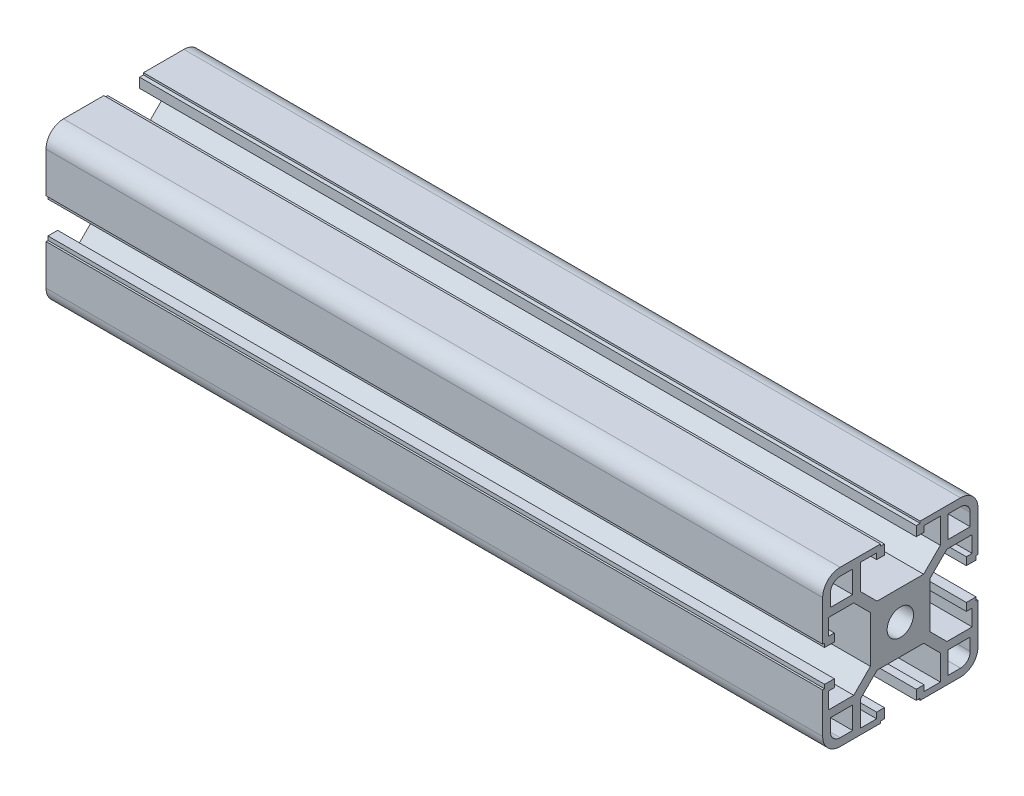
SolidWorks part; units mm, degrees
ref_plane "Front Plane" through (0, 0, 0) normal (0, 0, 1) x (1, 0, 0)
ref_plane "Top Plane" through (0, 0, 0) normal (0, 1, 0) x (1, 0, 0)
ref_plane "Right Plane" through (0, 0, 0) normal (1, 0, 0) x (0, 0, -1)
sketch "草图1" plane through (0, 0, 0) normal (0, 0, 1) x (1, 0, 0)
  line L0 (-984.975, 0) -> (-784.975, 0)
  dimension "D1" = 200
other "Aluminium profile 40 X 40B X R4.5(1)"
ref_plane "Plane1" through (-984.975, 0, 0) normal (1, 0, 0) x (0, 1, 0)
sketch "Sketch1" plane through (-984.975, 0, 0) normal (1, 0, 0) x (0, 1, 0)
  line L0 (-5.1, 20) -> (-5.1, 19.5)
  line L1 (-5.1, 19.5) -> (-4.1, 19.5)
  line L2 (-4.1, 19.5) -> (-4.1, 17)
  line L3 (-6.1, 18.5) -> (-10.3, 18.5)
  line L4 (-15.5, -20) -> (-5.1, -20)
  line L5 (-20, -15.5) -> (-20, -5.1)
  line L6 (15.5, 20) -> (5.1, 20)
  line L7 (20, 15.5) -> (20, 5.1)
  line L8 (0, 14.8756) -> (0, 0) construction
  line L9 (0, 0) -> (14.1675, 0) construction
  line L10 (-10.3, 18.5) -> (-10.3, 12)
  line L11 (-10.3, 12) -> (-6, 7.7)
  line L12 (-6, 7.7) -> (6, 7.7)
  line L13 (10.3, 12) -> (6, 7.7)
  line L14 (10.3, 18.5) -> (10.3, 12)
  line L15 (6.1, 18.5) -> (10.3, 18.5)
  line L16 (4.1, 19.5) -> (4.1, 17)
  line L17 (5.1, 19.5) -> (4.1, 19.5)
  line L18 (5.1, 20) -> (5.1, 19.5)
  line L19 (-5.1, 20) -> (-15.5, 20)
  line L20 (20, 5.1) -> (19.5, 5.1)
  line L21 (12.3, 18) -> (15.5, 18)
  line L22 (12.3, 18) -> (12.3, 12.3)
  line L23 (12.3, 12.3) -> (18, 12.3)
  line L24 (18, 15.5) -> (18, 12.3)
  line L25 (19.5, 5.1) -> (19.5, 4.1)
  line L26 (19.5, 4.1) -> (17, 4.1)
  line L27 (17, 6.1) -> (17, 4.1)
  line L28 (18.5, 6.1) -> (17, 6.1)
  line L29 (18.5, 6.1) -> (18.5, 10.3)
  line L30 (18.5, 10.3) -> (12, 10.3)
  line L31 (12, 10.3) -> (7.7, 6)
  line L32 (7.7, 6) -> (7.7, -6)
  line L33 (12, -10.3) -> (7.7, -6)
  line L34 (18.5, -10.3) -> (12, -10.3)
  line L35 (18.5, -6.1) -> (18.5, -10.3)
  line L36 (18.5, -6.1) -> (17, -6.1)
  line L37 (17, -4.1) -> (17, -6.1)
  line L38 (19.5, -4.1) -> (17, -4.1)
  line L39 (19.5, -5.1) -> (19.5, -4.1)
  line L40 (20, -5.1) -> (19.5, -5.1)
  line L41 (5.1, -20) -> (5.1, -19.5)
  line L42 (5.1, -19.5) -> (4.1, -19.5)
  line L43 (4.1, -19.5) -> (4.1, -17)
  line L44 (6.1, -17) -> (4.1, -17)
  line L45 (6.1, -18.5) -> (6.1, -17)
  line L46 (6.1, -18.5) -> (10.3, -18.5)
  line L47 (10.3, -18.5) -> (10.3, -12)
  line L48 (10.3, -12) -> (6, -7.7)
  line L49 (6, -7.7) -> (-6, -7.7)
  line L50 (-10.3, -12) -> (-6, -7.7)
  line L51 (-10.3, -18.5) -> (-10.3, -12)
  line L52 (-6.1, -18.5) -> (-10.3, -18.5)
  line L53 (-6.1, -18.5) -> (-6.1, -17)
  line L54 (-4.1, -17) -> (-6.1, -17)
  line L55 (-4.1, -19.5) -> (-4.1, -17)
  line L56 (-5.1, -19.5) -> (-4.1, -19.5)
  line L57 (-5.1, -20) -> (-5.1, -19.5)
  line L58 (-20, -5.1) -> (-19.5, -5.1)
  line L59 (5.1, -20) -> (15.5, -20)
  line L60 (-20, 5.1) -> (-20, 15.5)
  line L61 (-19.5, -5.1) -> (-19.5, -4.1)
  line L62 (-6.1, 18.5) -> (-6.1, 17)
  line L63 (-6.1, 17) -> (-4.1, 17)
  line L64 (6.1, 18.5) -> (6.1, 17)
  line L65 (4.1, 17) -> (6.1, 17)
  line L66 (-19.5, -4.1) -> (-17, -4.1)
  line L67 (-15.5, 18) -> (-12.3, 18)
  line L68 (-18, 15.5) -> (-18, 12.3)
  line L69 (-18, 12.3) -> (-12.3, 12.3)
  line L70 (-12.3, 18) -> (-12.3, 12.3)
  line L71 (-17, -6.1) -> (-17, -4.1)
  line L72 (-18.5, -6.1) -> (-17, -6.1)
  line L73 (-18.5, -6.1) -> (-18.5, -10.3)
  line L74 (-18.5, -10.3) -> (-12, -10.3)
  line L75 (-12, -10.3) -> (-7.7, -6)
  line L76 (-7.7, -6) -> (-7.7, 6)
  line L77 (-12, 10.3) -> (-7.7, 6)
  line L78 (-18.5, 10.3) -> (-12, 10.3)
  line L79 (-18.5, 6.1) -> (-18.5, 10.3)
  line L80 (-18.5, 6.1) -> (-17, 6.1)
  line L81 (-17, 4.1) -> (-17, 6.1)
  line L82 (-19.5, 4.1) -> (-17, 4.1)
  line L83 (-19.5, 5.1) -> (-19.5, 4.1)
  line L84 (-20, 5.1) -> (-19.5, 5.1)
  line L85 (20, -5.1) -> (20, -15.5)
  line L87 (-18, -12.3) -> (-12.3, -12.3)
  line L88 (-18, -12.3) -> (-18, -15.5)
  line L89 (-15.5, -18) -> (-12.3, -18)
  line L90 (-12.3, -12.3) -> (-12.3, -18)
  line L91 (12.3, -12.3) -> (18, -12.3)
  line L92 (12.3, -12.3) -> (12.3, -18)
  line L93 (12.3, -18) -> (15.5, -18)
  line L94 (18, -12.3) -> (18, -15.5)
  circle A0 centre (0, 0) radius 3.4
  arc A1 (-20, 15.5) -> (-15.5, 20) centre (-15.5, 15.5) cw
  arc A2 (20, 15.5) -> (15.5, 20) centre (15.5, 15.5) ccw
  arc A3 (-15.5, -20) -> (-20, -15.5) centre (-15.5, -15.5) cw
  arc A4 (15.5, -20) -> (20, -15.5) centre (15.5, -15.5) ccw
  arc A5 (-15.5, 18) -> (-18, 15.5) centre (-15.5, 15.5) ccw
  arc A6 (18, 15.5) -> (15.5, 18) centre (15.5, 15.5) ccw
  arc A7 (18, -15.5) -> (15.5, -18) centre (15.5, -15.5) cw
  arc A8 (-18, -15.5) -> (-15.5, -18) centre (-15.5, -15.5) ccw
  point P2 (0, 10)
  point P4 (0, 0)
  point P5 (-20, -20)
  point P6 (20, -20)
  point P7 (20, 20)
  point P8 (-20, 20)
  point P36 (-20, 20)
  point P39 (20, 20)
  point P121 (0, 0)
  dimension "D1" = 20.6
  dimension "D2" = 40
  dimension "D3" = 8.2
  dimension "D4" = 10.2
  dimension "D5" = 12.3
  dimension "D6" = 6.8
  dimension "D7" = 4.5
  dimension "D8" = 45
  dimension "D12" = 2
  dimension "D13" = 5.7
  dimension "D14" = 2
  dimension "D18" = 2.5
  dimension "D19" = 2.5
  dimension "D15" = 2.5
  dimension "D9" = 0.5
  dimension "D10" = 1.5
  dimension "D11" = 12
  dimension "D16" = 3
  dimension "D17" = 2
  dimension "D20" = 2
  dimension "D21" = 2
